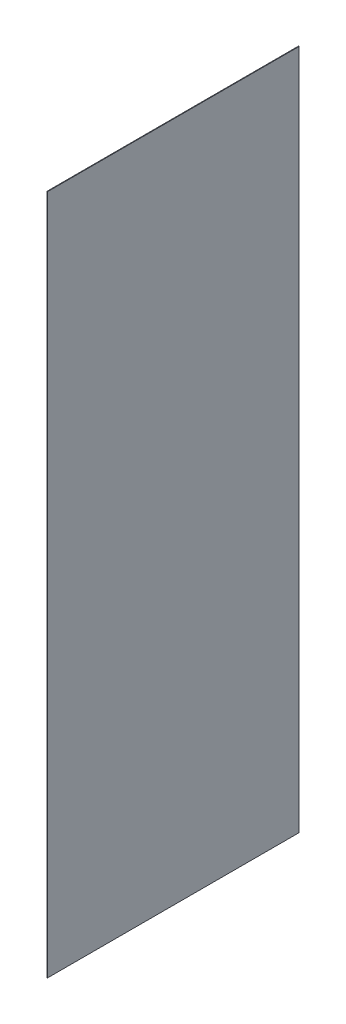
from build123d import *

# Parameters (mm, degrees)
SKETCH1_W           = 2124
SKETCH1_H           = 5744
BOSS_EXTRUDE1_DEPTH = 5


with BuildPart() as part:
    # Sketch1 → Boss-Extrude1 (new body)
    with BuildSketch(Plane.ZY.offset(95)):
        Rectangle(SKETCH1_W, SKETCH1_H)
    extrude(amount=BOSS_EXTRUDE1_DEPTH)


solid = part.part
